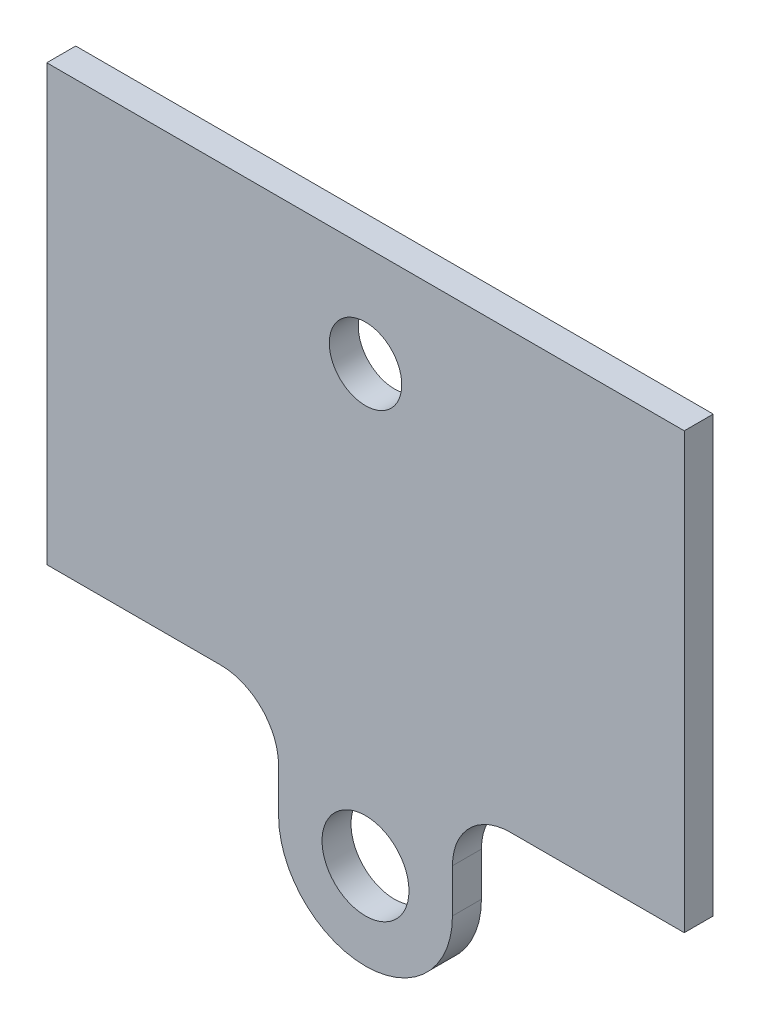
from build123d import *

# Parameters (mm, degrees)
SKETCH1_R           = 15
SKETCH1_R_2         = 12.5
BOSS_EXTRUDE1_DEPTH = 5
FILLET1_R           = 20


with BuildPart() as part:
    # Sketch1 → Boss-Extrude1 (new, symmetric)
    # profile 1 of 3: a face of its own
    with BuildSketch(Plane.XY):
        with BuildLine():
            Line((30, -110), (30, -75))
            Line((30, -75), (-30, -75))
            Line((-30, -75), (-30, -110))
            ThreePointArc((-30, -110), (0, -140), (30, -110))
        make_face()
        with Locations((0, -110)):
            Circle(SKETCH1_R, mode=Mode.SUBTRACT)
    # profile 2 of 3: a face of its own
    with BuildSketch(Plane.XY):
        with BuildLine():
            Line((30, -75), (110, -75))
            Line((110, -75), (110, 75))
            Line((110, 75), (-110, 75))
            Line((-110, 75), (-110, -75))
            Line((-110, -75), (-30, -75))
            ThreePointArc((-30, -75), (0, -45), (30, -75))
        make_face()
        with Locations((0, 40)):
            Circle(SKETCH1_R_2, mode=Mode.SUBTRACT)
    # profile 3 of 3: a face of its own
    with BuildSketch(Plane.XY):
        with BuildLine():
            Line((-30, -75), (30, -75))
            ThreePointArc((30, -75), (0, -45), (-30, -75))
        make_face()
    extrude(amount=BOSS_EXTRUDE1_DEPTH, both=True)

    # Fillet1
    fillet1_edges = [part.edges().sort_by_distance(p)[0] for p in [
        (-30, -75, 0),
        (30, -75, 0),
    ]]
    fillet(fillet1_edges, radius=FILLET1_R)


solid = part.part
